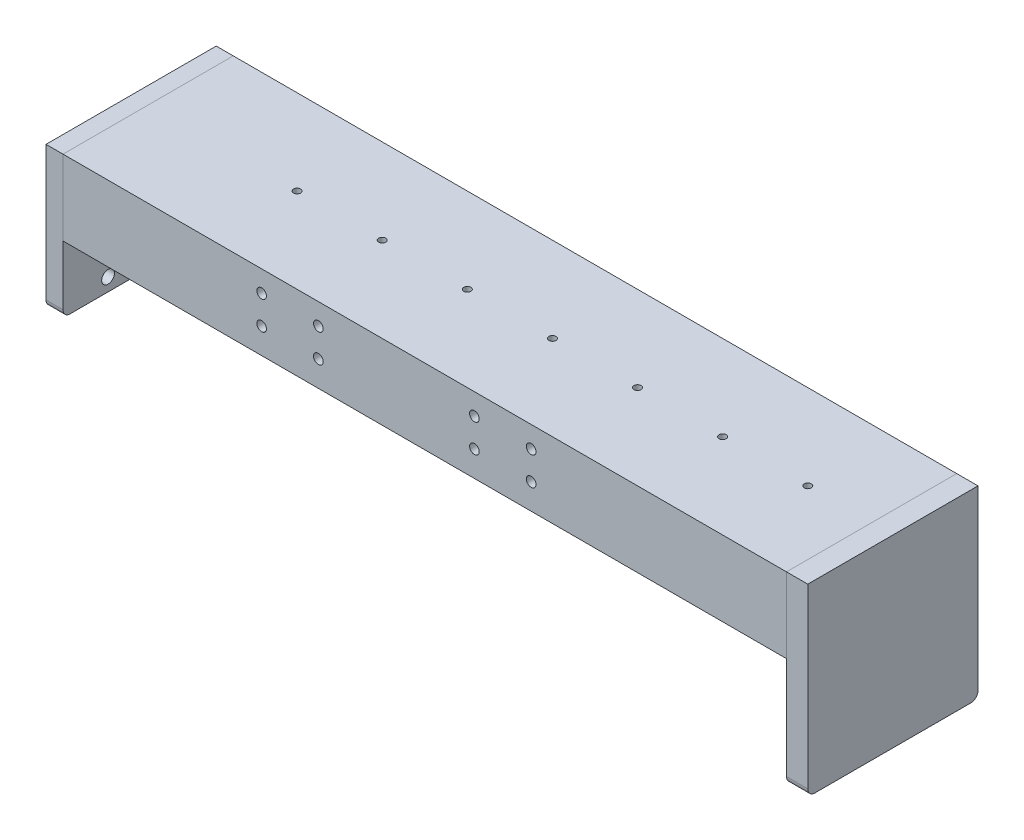
SolidWorks part; units mm, degrees
ref_plane "前视基准面" through (0, 0, 0) normal (0, 0, 1) x (1, 0, 0)
ref_plane "上视基准面" through (0, 0, 0) normal (0, 1, 0) x (1, 0, 0)
ref_plane "右视基准面" through (0, 0, 0) normal (1, 0, 0) x (0, 0, -1)
sketch "草图1" plane through (0, 0, 0) normal (0, 0, 1) x (1, 0, 0)
  line L0 (0, 0) -> (510, 0)
  dimension "D1" = 510
other "结构构件1"
ref_plane "基准面1" through (0, 0, 0) normal (1, 0, 0) x (0, 1, 0)
sketch "Sketch1" plane through (0, 0, 0) normal (1, 0, 0) x (0, 1, 0)
  line L0 (0, 0) -> (0, -120)
  line L1 (0, -120) -> (-53, -120)
  line L2 (0, -60) -> (-5.5, -60) construction
  line L3 (-5.5, -101.1579) -> (-5.5, -18.8421)
  line L4 (-13.8856, -110.1369) -> (-48.8072, -112.5263)
  line L5 (-53, -117.0158) -> (-53, -120)
  line L6 (-5.5, -109.5632) -> (-5.5, -112.8132) construction
  line L7 (-5.5, -112.8132) -> (-53, -112.8132) construction
  line L8 (-26.5, -120) -> (-26.5, -111) construction
  line L9 (-53, -2.9842) -> (-53, 0)
  line L10 (0, 0) -> (-53, 0)
  line L11 (-13.8856, -9.8631) -> (-48.8072, -7.4737)
  arc A0 (-5.5, -101.1579) -> (-13.8856, -110.1369) centre (-14.5, -101.1579) cw
  arc A1 (-13.8856, -9.8631) -> (-5.5, -18.8421) centre (-14.5, -18.8421) cw
  arc A2 (-48.8072, -112.5263) -> (-53, -117.0158) centre (-48.5, -117.0158) ccw
  arc A3 (-53, -2.9842) -> (-48.8072, -7.4737) centre (-48.5, -2.9842) ccw
  point P2 (-26.5, 0)
  point P17 (0, 0)
  point P20 (-5.5, -10.4368)
  point P26 (-53, -7.1868)
  dimension "r" = 9
  dimension "r1" = 4.5
  dimension "h" = 120
  dimension "b" = 53
  dimension "d" = 5.5
  dimension "x" = 9
  dimension "D5" = 47.5
  dimension "D6" = 3.25
sketch "草图5" plane through (0, 0, 0) normal (-1, 0, 0) x (0, 0, 1)
  line L0 (0, 0) -> (0, -53) construction
  line L1 (-120, 0) -> (0, 0)
  line L2 (-120, 0) -> (-120, -100)
  line L3 (-120, -100) -> (0, -100)
  line L4 (0, 0) -> (0, -100)
  dimension "D1" = 100
extrude "凸台-拉伸1" add sketch "草图5" along normal blind 12 separate body
sketch "草图6" plane through (510, 0, 0) normal (1, 0, 0) x (0, 0, -1)
  line L0 (0, 0) -> (0, -53) construction
  line L1 (120, 0) -> (0, 0)
  line L2 (120, 0) -> (120, -130)
  line L3 (120, -130) -> (0, -130)
  line L4 (0, 0) -> (0, -130)
  dimension "D1" = 130
extrude "凸台-拉伸2" add sketch "草图6" along normal blind 15 separate body
fillet "圆角1" radius 5 2 edges at (-6, -100, 0) (-6, -100, -120)
fillet "圆角2" radius 5 2 edges at (517.5, -130, 0) (517.5, -130, -120)
hole_wizard "M6 螺纹孔1" positions "草图8" profile "草图7" tap size "M6" standard "GB"
sketch "草图8" plane through (0, -5.5, 0) normal (0, -1, 0) x (-1, 0, 0)
  point P0 (-105, 60)
  point P3 (-165, 60)
  point P6 (-225, 60)
  point P9 (-285, 60)
  point P12 (-345, 60)
  point P15 (-405, 60)
  point P18 (-465, 60)
sketch "草图7" plane through (105, -5.5, -60) normal (1, 0, 0) x (0, 0, -1)
  line L0 (0, 0) -> (0, 16.5022)
  line L1 (0, 16.5022) -> (2.5, 15)
  line L2 (2.5, 15) -> (2.5, 0)
  line L5 (2.5, 0) -> (0, 0)
  line L10 (0, 16.5022) -> (-2.5, 15) construction
  line L11 (0, -6.35) -> (0, 107.95) construction
  dimension "螺纹孔钻头直径" = 5
  dimension "螺纹孔钻头深度" = 15
  dimension "导头角度" = 118
cosmetic thread "孔螺蚊线1" parameters "D1"=5.5, "D2"=6
cosmetic thread "孔螺蚊线2" parameters "D1"=5.5, "D2"=6
cosmetic thread "孔螺蚊线3" parameters "D1"=5.5, "D2"=6
cosmetic thread "孔螺蚊线4" parameters "D1"=5.5, "D2"=6
cosmetic thread "孔螺蚊线5" parameters "D1"=5.5, "D2"=6
cosmetic thread "孔螺蚊线6" parameters "D1"=5.5, "D2"=6
cosmetic thread "孔螺蚊线7" parameters "D1"=5.5, "D2"=6
hole_wizard "M8 螺纹孔1" positions "草图10" profile "草图9" tap size "M8" standard "GB"
sketch "草图10" plane through (0, -130, 0) normal (0, -1, 0) x (-1, 0, 0)
  line L0 (-517.5, 115) -> (-517.5, 5) construction
  line L1 (-510, 115) -> (-525, 115) construction
  line L2 (-525, 5) -> (-510, 5) construction
  line L4 (-510, 60) -> (-525, 60) construction
  line L5 (-510, 5) -> (-510, 115) construction
  line L6 (-525, 5) -> (-525, 115) construction
  point P0 (-517.5, 100)
  point P2 (-517.5, 20)
  point P23 (-517.5, 60)
  dimension "D1" = 80
sketch "草图9" plane through (517.5, -130, -100) normal (1, 0, 0) x (0, 0, -1)
  line L0 (0, 0) -> (0, 21.7929)
  line L1 (0, 21.7929) -> (3.4, 19.75)
  line L2 (3.4, 19.75) -> (3.4, 0)
  line L5 (3.4, 0) -> (0, 0)
  line L10 (0, 21.7929) -> (-3.4, 19.75) construction
  line L11 (0, -6.35) -> (0, 107.95) construction
  dimension "螺纹孔钻头直径" = 6.8
  dimension "螺纹孔钻头深度" = 19.75
  dimension "导头角度" = 118
cosmetic thread "孔螺蚊线8" parameters "D1"=16, "D2"=8
cosmetic thread "孔螺蚊线9" parameters "D1"=16, "D2"=8
cosmetic thread "孔螺蚊线10" parameters "D1"=16, "D2"=8
hole_wizard "M8 螺纹孔2" positions "草图12" profile "草图11" tap size "M8" standard "GB" end condition through all
sketch "草图12" plane through (0, 0, -120) normal (0, 0, -1) x (-1, 0, 0)
  line L0 (0, 0) -> (-510, 0) construction
  line L1 (0, 0) -> (0, -95) construction
  point P0 (-140, -15)
  point P3 (-140, -35)
  point P6 (-180, -35)
  point P9 (-180, -15)
  dimension "D1" = 40
  dimension "D2" = 20
  dimension "D3" = 15
  dimension "D4" = 140
cosmetic thread "孔螺蚊线11" parameters "D2"=8
cosmetic thread "孔螺蚊线12" parameters "D2"=8
cosmetic thread "孔螺蚊线13" parameters "D2"=8
cosmetic thread "孔螺蚊线14" parameters "D2"=8
sketch "草图11" plane through (140, -15, -120) normal (1, 0, 0) x (0, 1, 0)
  line L0 (0, 0) -> (0, 120)
  line L1 (0, 120) -> (3.4, 120)
  line L2 (3.4, 120) -> (3.4, 0)
  line L5 (3.4, 0) -> (0, 0)
  line L11 (0, -6.35) -> (0, 107.95) construction
  dimension "通孔螺纹孔钻头直径" = 6.8
  dimension "通孔螺纹孔钻头深度" = 120
hole_wizard "Ø9.0 (9) 直径孔1" positions "草图14" profile "草图13" hole size "Ø9.0" standard "GB"
sketch "草图14" plane through (0, 0, 0) normal (1, 0, 0) x (0, 0, -1)
  point P0 (31.75, -90.75)
  point P3 (31.75, -34.25)
  point P6 (88.25, -34.25)
  point P9 (88.25, -90.75)
sketch "草图13" plane through (0, -90.75, -31.75) normal (0, 1, 0) x (0, 0, -1)
  line L0 (0, 0) -> (0, 22.7039)
  line L1 (0, 22.7039) -> (4.5, 20)
  line L2 (4.5, 20) -> (4.5, 0)
  line L5 (4.5, 0) -> (0, 0)
  line L10 (0, 22.7039) -> (-4.5, 20) construction
  line L11 (0, -6.35) -> (0, 107.95) construction
  dimension "孔直径" = 9
  dimension "孔深度" = 20
  dimension "导头角度" = 118
sketch "草图15" plane through (0, 0, 0) normal (1, 0, 0) x (0, 0, -1)
  circle A0 centre (60, -62.5) radius 25
  dimension "D1" = 50
extrude "切除-拉伸1" cut sketch "草图15" against normal blind 20
pattern_linear "阵列(线性)1" count 2 spacing 150 along (1, 0, 0) of "M8 螺纹孔2"
